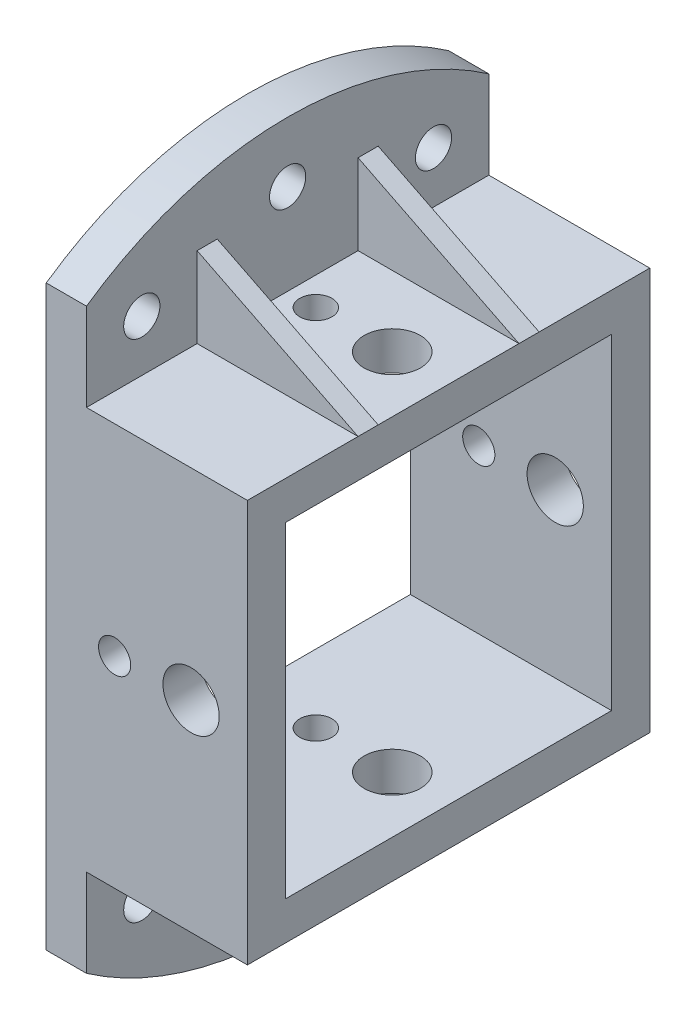
SolidWorks part; units mm, degrees
material "普通碳钢"
ref_plane "Front Plane" through (0, 0, 0) normal (0, 0, 1) x (1, 0, 0)
ref_plane "Top Plane" through (0, 0, 0) normal (0, 1, 0) x (1, 0, 0)
ref_plane "Right Plane" through (0, 0, 0) normal (1, 0, 0) x (0, 0, -1)
sketch "Sketch4" plane through (0, 0, 0) normal (1, 0, 0) x (0, 0, -1)
  line L0 (50, 50) -> (-50, 50)
  line L1 (40.5, -40.5) -> (-40.5, -40.5)
  line L2 (40.5, -40.5) -> (40.5, 40.5)
  line L3 (40.5, 40.5) -> (-40.5, 40.5)
  line L4 (-40.5, -40.5) -> (-40.5, 40.5)
  line L5 (40.5, -40.5) -> (-40.5, 40.5) construction
  line L6 (40.5, 40.5) -> (-40.5, -40.5) construction
  line L7 (-50, -50) -> (-50, 50)
  line L8 (50, -50) -> (-50, -50)
  line L9 (50, -50) -> (50, 50)
  line L10 (34.5, -40.5) -> (-34.5, -40.5) construction
  line L11 (-40.5, -34.5) -> (-40.5, 34.5) construction
  line L12 (34.5, 40.5) -> (-34.5, 40.5) construction
  line L13 (40.5, -34.5) -> (40.5, 34.5) construction
  line L14 (34.5, -50) -> (-34.5, -50) construction
  line L15 (-50, -34.5) -> (-50, 34.5) construction
  line L16 (50, -34.5) -> (50, 34.5) construction
  line L17 (34.5, 50) -> (-34.5, 50) construction
  arc A8 (-34.5, -50) -> (-50, -34.5) centre (-34.5, -34.5) cw construction
  arc A9 (34.5, -50) -> (50, -34.5) centre (34.5, -34.5) ccw construction
  arc A10 (50, 34.5) -> (34.5, 50) centre (34.5, 34.5) ccw construction
  arc A11 (-34.5, 50) -> (-50, 34.5) centre (-34.5, 34.5) ccw construction
  arc A12 (-34.5, -40.5) -> (-40.5, -34.5) centre (-34.5, -34.5) cw construction
  arc A13 (34.5, -40.5) -> (40.5, -34.5) centre (34.5, -34.5) ccw construction
  arc A14 (40.5, 34.5) -> (34.5, 40.5) centre (34.5, 34.5) ccw construction
  arc A15 (-34.5, 40.5) -> (-40.5, 34.5) centre (-34.5, 34.5) ccw construction
  point P0 (0, 0)
  dimension "D1" = 81
  dimension "D2" = 81
  dimension "D4" = 9.5
extrude "Boss-Extrude1" add sketch "Sketch4" along normal blind 40
sketch "Sketch5" plane through (0, 0, 0) normal (-1, 0, 0) x (0, 0, 1)
  circle A0 centre (0, 0) radius 87.5
  dimension "D1" = 175
extrude "Boss-Extrude2" add sketch "Sketch5" along normal blind 10
sketch "Sketch6" plane through (-10, 0, 0) normal (-1, 0, 0) x (0, 0, 1)
  line L1 (50, -106.3756) -> (-50, -106.3756)
  line L2 (50, -106.3756) -> (50, 106.3756)
  line L3 (50, 106.3756) -> (-50, 106.3756)
  line L4 (-50, -106.3756) -> (-50, 106.3756)
  line L5 (50, -106.3756) -> (-50, 106.3756) construction
  line L6 (50, 106.3756) -> (-50, -106.3756) construction
  point P0 (0, 0)
  dimension "D1" = 100
  dimension "D2" = 212.7511
extrude "Cut-Extrude1" cut sketch "Sketch6" against normal blind 10 flip side to cut
sketch "Sketch7" plane through (0, 0, 0) normal (1, 0, 0) x (0, 0, -1)
  line L0 (40.5, -40.5) -> (40.5, 40.5) construction
  line L1 (-40.5, -40.5) -> (40.5, -40.5) construction
  line L2 (-40.5, 40.5) -> (-40.5, -40.5) construction
  line L3 (40.5, 40.5) -> (-40.5, 40.5) construction
  line L4 (40.5, -40.5) -> (40.5, 40.5)
  line L5 (-40.5, -40.5) -> (40.5, -40.5)
  line L6 (-40.5, 40.5) -> (-40.5, -40.5)
  line L7 (40.5, 40.5) -> (-40.5, 40.5)
extrude "Cut-Extrude2" cut sketch "Sketch7" against normal blind 10
sketch "Sketch8" plane through (0, 0, 0) normal (1, 0, 0) x (0, 0, -1)
  line L0 (0, 0) -> (-36.25, 62.7868) construction
  line L1 (0, 0) -> (0, 72.5) construction
  line L2 (-40.5, 0) -> (40.5, 0) construction
  line L3 (-40.5, 40.5) -> (-40.5, -40.5) construction
  line L4 (40.5, -40.5) -> (40.5, 40.5) construction
  circle A0 centre (0, 0) radius 72.5 construction
  circle A1 centre (-36.25, 62.7868) radius 4.5
  circle A2 centre (0, 72.5) radius 4.5
  circle A3 centre (36.25, 62.7868) radius 4.5
  circle A13 centre (36.25, -62.7868) radius 4.5
  circle A14 centre (0, -72.5) radius 4.5
  circle A15 centre (-36.25, -62.7868) radius 4.5
  point P30 (0, 0)
  dimension "D1" = 145
  dimension "D2" = 9
  dimension "D3" = 30
extrude "Cut-Extrude3" cut sketch "Sketch8" against normal blind 10
hole_wizard "M16 Tapped Hole1" positions "Sketch9" profile "Sketch10" tap size "M16" standard "GB" end condition through all
sketch "Sketch9" plane through (0, 0, 50) normal (0, 0, 1) x (1, 0, 0)
  line L0 (40, 50) -> (40, -50) construction
  point P0 (26, 0)
  dimension "D1" = 14
sketch "Sketch10" plane through (26, 0, 50) normal (1, 0, 0) x (0, -1, 0)
  line L0 (0, 0) -> (0, 100)
  line L1 (0, 100) -> (7, 100)
  line L2 (7, 100) -> (7, 0)
  line L5 (7, 0) -> (0, 0)
  line L11 (0, -6.35) -> (0, 107.95) construction
  dimension "通孔螺纹孔钻头直径" = 14
  dimension "通孔螺纹孔钻头深度" = 100
cosmetic thread "Hole Thread Line1" parameters "D2"=16
hole_wizard "M16 Tapped Hole2" positions "Sketch11" profile "Sketch12" tap size "M16" standard "GB" end condition through all
sketch "Sketch11" plane through (0, 50, 0) normal (0, 1, 0) x (1, 0, 0)
  line L0 (40, 50) -> (40, -50) construction
  point P0 (26, 0)
  dimension "D1" = 14
sketch "Sketch12" plane through (26, 50, 0) normal (1, 0, 0) x (0, 0, 1)
  line L0 (0, 0) -> (0, 137.5)
  line L1 (0, 137.5) -> (7, 137.5)
  line L2 (7, 137.5) -> (7, 0)
  line L5 (7, 0) -> (0, 0)
  line L11 (0, -6.35) -> (0, 107.95) construction
  dimension "通孔螺纹孔钻头直径" = 14
  dimension "通孔螺纹孔钻头深度" = 137.5
cosmetic thread "Hole Thread Line2" parameters "D2"=16
hole_wizard "Size mm Dowel Hole2" positions "Sketch13" profile "Sketch14" hole size "Ø8.0" standard "GB" end condition through all
sketch "Sketch13" plane through (0, 0, 50) normal (0, 0, 1) x (1, 0, 0)
  circle A0 centre (26, 0) radius 7 construction
  point P0 (7, 0)
  dimension "D1" = 19
sketch "Sketch14" plane through (7, 0, 50) normal (1, 0, 0) x (0, -1, 0)
  line L0 (0, 0) -> (0, 100)
  line L1 (0, 100) -> (4, 100)
  line L2 (4, 100) -> (4, 0)
  line L5 (4, 0) -> (0, 0)
  line L11 (0, -6.35) -> (0, 107.95) construction
  dimension "通孔孔直径" = 8
  dimension "通孔孔深度" = 100
hole_wizard "大小mm 暗销孔2" positions "Sketch15" profile "Sketch16" hole size "Ø8.0" standard "GB" end condition through all
sketch "Sketch15" plane through (0, 50, 0) normal (0, 1, 0) x (1, 0, 0)
  circle A0 centre (26, 0) radius 7 construction
  point P0 (7, 0)
  dimension "D1" = 19
sketch "Sketch16" plane through (7, 50, 0) normal (1, 0, 0) x (0, 0, 1)
  line L0 (0, 0) -> (0, 137.5)
  line L1 (0, 137.5) -> (4, 137.5)
  line L2 (4, 137.5) -> (4, 0)
  line L5 (4, 0) -> (0, 0)
  line L11 (0, -6.35) -> (0, 107.95) construction
  dimension "通孔孔直径" = 8
  dimension "通孔孔深度" = 137.5
ref_plane "Plane1" through (0, 0, 20) normal (0, 0, 1) x (1, 0, 0)
sketch "Sketch18" plane through (0, 0, 20) normal (0, 0, 1) x (1, 0, 0)
  line L0 (40, 50) -> (0, 70)
  line L1 (0, 71.807) -> (0, 87.5) construction
  line L3 (40, 0) -> (-10, 0) construction
  line L4 (40, 50) -> (40, -50) construction
  line L5 (-10, -71.807) -> (-10, 71.807) construction
  line L6 (40, 50) -> (0, 50) construction
  dimension "D1" = 20
rib "Rib2" sketch "Sketch18" sketch "Sketch18" thickness 5 extrusion direction parallel to sketch draft on no parameters "D1"=5
mirror "Mirror1" about plane through (0, 0, 0) normal (0, 1, 0) of "Rib2"
mirror "Mirror2" about plane through (0, 0, 0) normal (0, 0, 1) of "Mirror1", "Rib2"
